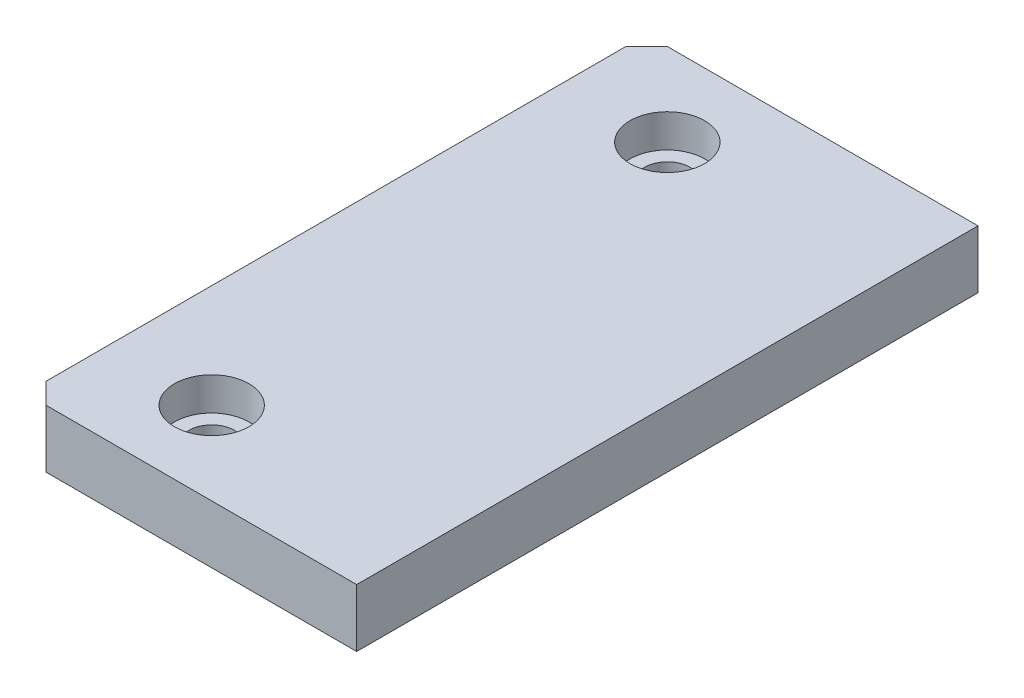
SolidWorks part; units mm, degrees
material "Q235"
ref_plane "Front Plane" through (0, 0, 0) normal (0, 0, 1) x (1, 0, 0)
ref_plane "Top Plane" through (0, 0, 0) normal (0, 1, 0) x (1, 0, 0)
ref_plane "Right Plane" through (0, 0, 0) normal (1, 0, 0) x (0, 0, -1)
sketch "Sketch1" plane through (0, 0, 0) normal (0, 1, 0) x (1, 0, 0)
  line L1 (0, 0) -> (80, 0)
  line L2 (0, 0) -> (0, 150)
  line L3 (0, 150) -> (80, 150)
  line L4 (80, 0) -> (80, 150)
  dimension "D1" = 150
  dimension "D2" = 80
extrude "Boss-Extrude1" add sketch "Sketch1" along normal blind 14
hole_wizard "Hole size (by socket head cap screw type)1" positions "Sketch2" profile "Sketch3" counterbore size "M10" standard "GB" end condition through all
sketch "Sketch2" plane through (0, 14, 0) normal (0, 1, 0) x (1, 0, 0)
  line L3 (80, 75) -> (0, 75) construction
  line L4 (80, 0) -> (80, 150) construction
  line L5 (0, 150) -> (0, 0) construction
  point P2 (25, 130)
  point P4 (25, 20)
  dimension "D1" = 25
  dimension "D2" = 110
sketch "Sketch3" plane through (25, 14, -130) normal (1, 0, 0) x (0, 0, 1)
  line L0 (0, 0) -> (0, 14)
  line L1 (0, 14) -> (5.5, 14)
  line L3 (5.5, 14) -> (5.5, 8)
  line L4 (5.5, 8) -> (9, 8)
  line L5 (9, 8) -> (9, 0)
  line L7 (9, 0) -> (0, 0)
  line L11 (0, -6.35) -> (0, 107.95) construction
  dimension "通孔孔直径" = 11
  dimension "通孔孔深度" = 14
  dimension "柱形沉头孔直径" = 18
  dimension "柱形沉头孔深度" = 8
chamfer "Chamfer1" distance 5 angle 45 2 edges at (0, 7, 0) (0, 7, -150)
